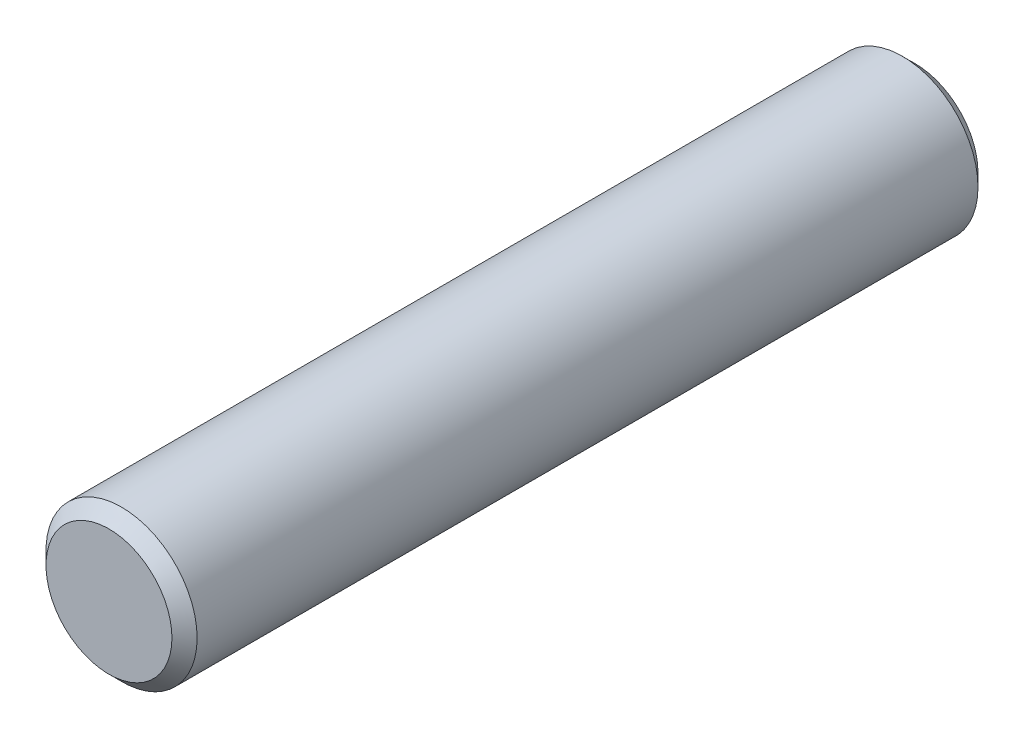
from build123d import *

# Parameters (mm, degrees)
SKETCH_1_R      = 3
EXTRUDE_1_DEPTH = 32
CHAMFER_1_SIZE  = 0.5


with BuildPart() as part:
    # 草图1 → 凸台-拉伸1 (new body)
    with BuildSketch(Plane.XY):
        Circle(SKETCH_1_R)
    extrude(amount=EXTRUDE_1_DEPTH)

    # 倒角1
    chamfer_1_edges = [part.edges().sort_by_distance(p)[0] for p in [
        (-3, 0, 0),
        (-3, 0, 32),
    ]]
    chamfer(chamfer_1_edges, length=CHAMFER_1_SIZE)


solid = part.part
